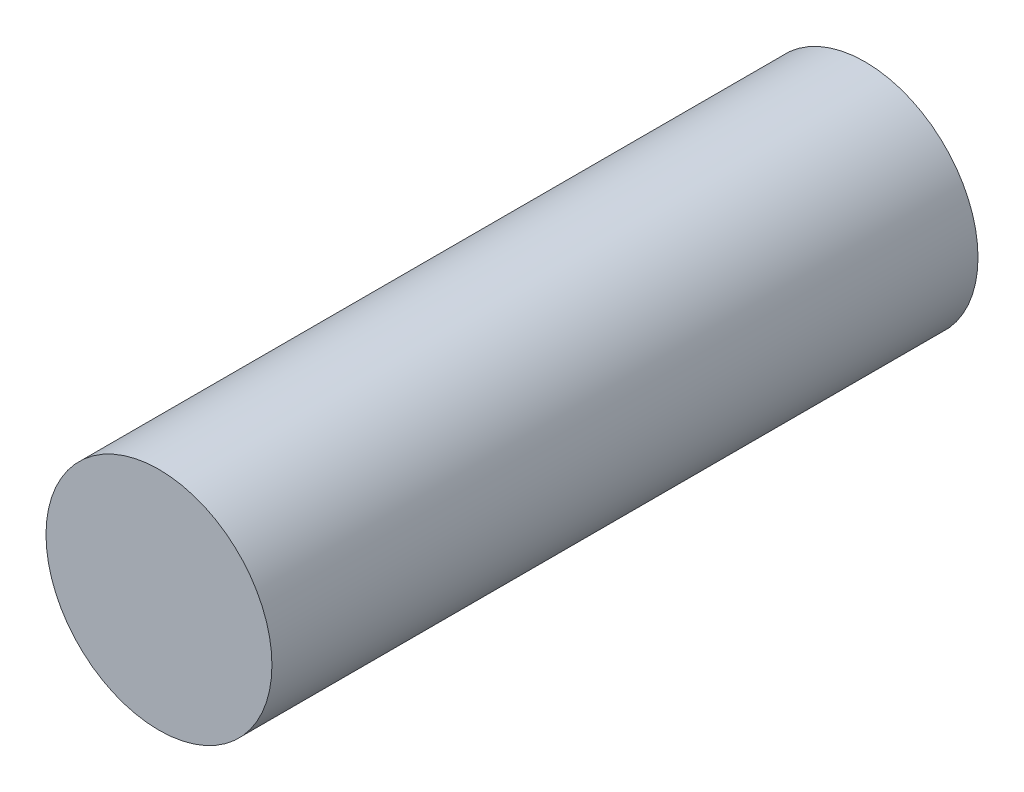
from build123d import *

# Parameters (mm, degrees)
SKETCH1_R           = 4
BOSS_EXTRUDE1_DEPTH = 25


with BuildPart() as part:
    # Sketch1 → Boss-Extrude1 (new body)
    with BuildSketch(Plane.XY):
        Circle(SKETCH1_R)
    extrude(amount=BOSS_EXTRUDE1_DEPTH)


solid = part.part
